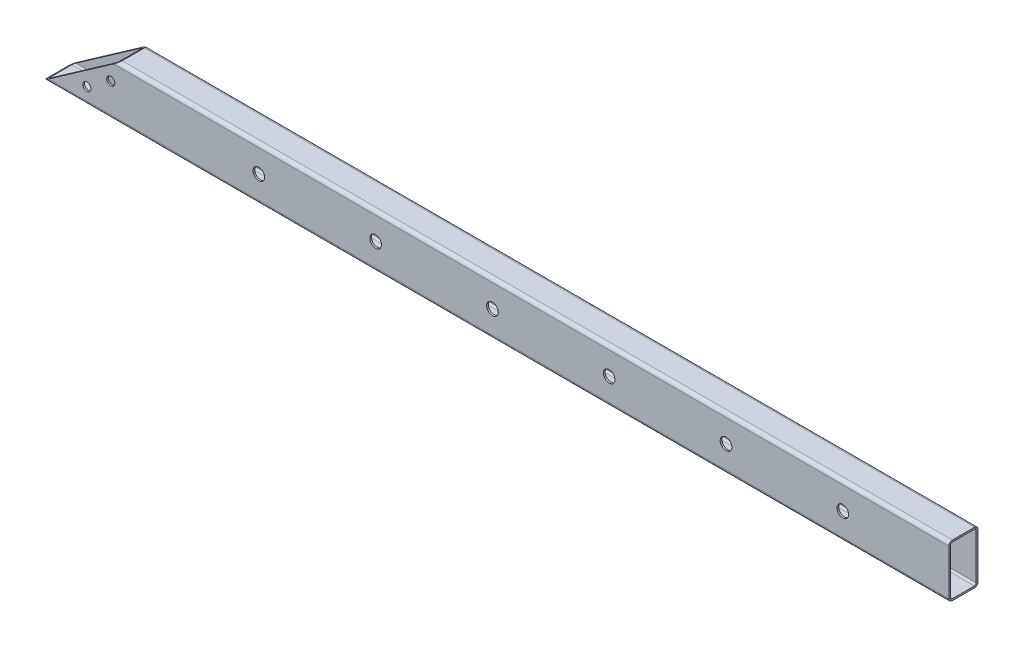
SolidWorks part; units mm, degrees
material "普通碳钢"
ref_plane "前视基准面" through (0, 0, 0) normal (0, 0, 1) x (1, 0, 0)
ref_plane "上视基准面" through (0, 0, 0) normal (0, 1, 0) x (1, 0, 0)
ref_plane "右视基准面" through (0, 0, 0) normal (1, 0, 0) x (0, 0, -1)
sketch "草图1" plane through (0, 0, 0) normal (0, 0, 1) x (1, 0, 0)
  line L0 (0, 0) -> (1550, 0)
  dimension "D1" = 1550
other "冷弯空心矩管gb∕t6728-2002 90 X 50 X 4(1)"
ref_plane "基准面1" through (0, 0, 0) normal (1, 0, 0) x (0, 0, 1)
sketch "Sketch11" plane through (0, 0, 0) normal (1, 0, 0) x (0, 0, 1)
  line L0 (-19, -42) -> (19, -42)
  line L1 (-22, -39) -> (-22, 39)
  line L2 (19, 42) -> (-19, 42)
  line L3 (22, 39) -> (22, -39)
  line L4 (-19, -45) -> (19, -45)
  line L5 (-25, -39) -> (-25, 39)
  line L6 (19, 45) -> (-19, 45)
  line L7 (25, 39) -> (25, -39)
  arc A0 (25, 39) -> (19, 45) centre (19, 39) ccw
  arc A1 (19, -45) -> (25, -39) centre (19, -39) ccw
  arc A2 (-25, -39) -> (-19, -45) centre (-19, -39) ccw
  arc A3 (-19, 45) -> (-25, 39) centre (-19, 39) ccw
  arc A4 (-19, 42) -> (-22, 39) centre (-19, 39) ccw
  arc A5 (22, 39) -> (19, 42) centre (19, 39) ccw
  arc A6 (19, -42) -> (22, -39) centre (19, -39) ccw
  arc A7 (-22, -39) -> (-19, -42) centre (-19, -39) ccw
  point P0 (0, 45)
  point P1 (25, 0)
  point P2 (0, -45)
  point P3 (-25, 0)
  point P4 (-25, 45)
  point P5 (25, 45)
  point P6 (25, -45)
  point P7 (-25, -45)
  point P8 (0, 0)
  point P33 (0, 0)
  dimension "D1" = 6
  dimension "Thickness" = 3
  dimension "V_leg" = 90
  dimension "H_leg" = 50
ref_plane "基准面2" through (21.1431, -30.1955, 0) normal (0.5736, -0.8192, 0) x (0, 0, -1)
split "分割1" trim tools "基准面2" bodies to split 106 resulting bodies 110
hole_wizard "Ø20.0 (20) 直径孔1" positions "草图3" profile "草图4" hole size "Ø20.0" standard "ISO"
sketch "草图3" plane through (0, 0, 25) normal (0, 0, 1) x (1, 0, 0)
  point P0 (368.5333, 0)
  dimension "D1" = 240
sketch "草图4" plane through (368.5333, 0, 25) normal (1, 0, 0) x (0, -1, 0)
  line L0 (0, 0) -> (0, 56.0076)
  line L1 (0, 56.0076) -> (10, 49.999)
  line L2 (10, 49.999) -> (10, 0)
  line L5 (10, 0) -> (0, 0)
  line L10 (0, 56.0076) -> (-10, 49.999) construction
  line L11 (0, -6.35) -> (0, 107.95) construction
  dimension "孔直径" = 20
  dimension "孔深度" = 49.999
  dimension "导头角度" = 118
pattern_linear "阵列(线性)1" count 6 spacing 200 along (1, 0, 0) of "Ø20.0 (20) 直径孔1"
hole_wizard "Ø14.0 (14) 直径孔2" positions "草图8" profile "草图9" hole size "Ø14.0" standard "ISO"
sketch "草图8" plane through (0, 0, 25) normal (0, 0, 1) x (1, 0, 0)
  point P0 (115.0285, 11.1283)
  point P3 (74.0709, -17.5505)
sketch "草图9" plane through (115.0285, 11.1283, 25) normal (1, 0, 0) x (0, -1, 0)
  line L0 (0, 0) -> (0, 54.205)
  line L1 (0, 54.205) -> (7, 49.999)
  line L2 (7, 49.999) -> (7, 0)
  line L5 (7, 0) -> (0, 0)
  line L10 (0, 54.205) -> (-7, 49.999) construction
  line L11 (0, -6.35) -> (0, 107.95) construction
  dimension "孔直径" = 14
  dimension "孔深度" = 49.999
  dimension "导头角度" = 118
